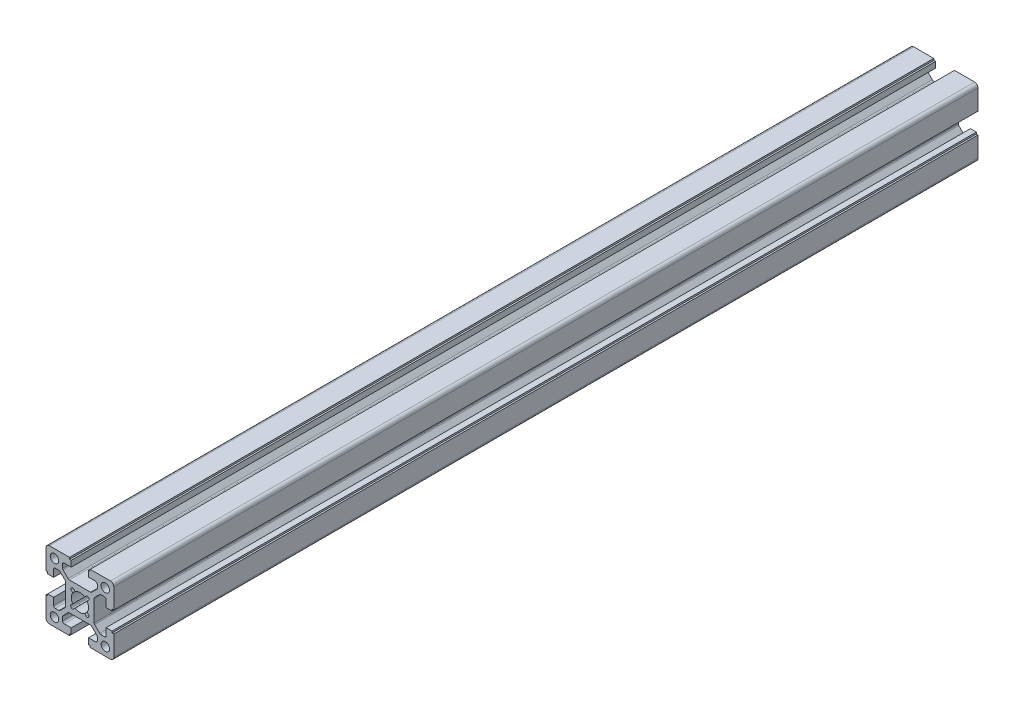
from build123d import *

# Parameters (mm, degrees)
SKETCH1_R           = 2.5
BOSS_EXTRUDE1_DEPTH = 255


with BuildPart() as part:
    # Sketch1 → Boss-Extrude1 (new, symmetric)
    with BuildSketch(Plane.XY):
        with BuildLine():
            Line((-5.1005, 15.500896213), (-5.1005, 19.000896213))
            Line((-5.1005, 19.000896213), (-6.1005, 19.000896213))
            Line((-6.1005, 19.000896213), (-6.1005, 20.000896213))
            Line((-6.1005, 20.000896213), (-18.0005, 20.000896213))
            ThreePointArc((-18.0005, 20.000896213), (-19.414713562, 19.415109775), (-20.0005, 18.000896213))
            Line((-20.0005, 18.000896213), (-20.0005, 6.100896213))
            Line((-20.0005, 6.100896213), (-19.0005, 6.100896213))
            Line((-19.0005, 6.100896213), (-19.0005, 5.100896213))
            Line((-19.0005, 5.100896213), (-15.5005, 5.100896213))
            Line((-15.5005, 5.100896213), (-15.5005, 9.250896213))
            ThreePointArc((-15.5005, 9.250896213), (-15.207606781, 9.958002994), (-14.5005, 10.250896213))
            Line((-14.5005, 10.250896213), (-12.431713562, 10.250896213))
            ThreePointArc((-12.431713562, 10.250896213), (-12.049030228, 10.174775786), (-11.724606932, 9.958003144))
            Line((-11.724606932, 9.958003144), (-8.693393219, 6.926789431))
            ThreePointArc((-8.693393219, 6.926789431), (-8.476620546, 6.602366272), (-8.4005, 6.21968306))
            Line((-8.4005, 6.21968306), (-8.4005, -6.217890225))
            ThreePointArc((-8.4005, -6.217890225), (-8.476620502, -6.60057374), (-8.693393346, -6.924997133))
            Line((-8.693393346, -6.924997133), (-11.724606781, -9.956210569))
            ThreePointArc((-11.724606781, -9.956210569), (-12.049030198, -10.172983348), (-12.431713709, -10.249103787))
            Line((-12.431713709, -10.249103787), (-14.5005, -10.249103787))
            ThreePointArc((-14.5005, -10.249103787), (-15.207606781, -9.956210569), (-15.5005, -9.249103787))
            Line((-15.5005, -9.249103787), (-15.5005, -5.099103787))
            Line((-15.5005, -5.099103787), (-19.0005, -5.099103787))
            Line((-19.0005, -5.099103787), (-19.0005, -6.099103787))
            Line((-19.0005, -6.099103787), (-20.0005, -6.099103787))
            Line((-20.0005, -6.099103787), (-20.0005, -17.999103787))
            ThreePointArc((-20.0005, -17.999103787), (-19.414713562, -19.41331735), (-18.0005, -19.999103787))
            Line((-18.0005, -19.999103787), (-6.1005, -19.999103787))
            Line((-6.1005, -19.999103787), (-6.1005, -18.999103787))
            Line((-6.1005, -18.999103787), (-5.1005, -18.999103787))
            Line((-5.1005, -18.999103787), (-5.1005, -15.499103787))
            Line((-5.1005, -15.499103787), (-9.2505, -15.499103787))
            ThreePointArc((-9.2505, -15.499103787), (-9.957606781, -15.206210569), (-10.2505, -14.499103787))
            Line((-10.2505, -14.499103787), (-10.2505, -12.43131735))
            ThreePointArc((-10.2505, -12.43131735), (-10.174379535, -12.048633922), (-9.957606789, -11.724210576))
            Line((-9.957606789, -11.724210576), (-6.925393219, -8.691997006))
            ThreePointArc((-6.925393219, -8.691997006), (-6.60096987, -8.475224255), (-6.218286438, -8.399103787))
            Line((-6.218286438, -8.399103787), (6.218286438, -8.399103787))
            ThreePointArc((6.218286438, -8.399103787), (6.600969772, -8.475224214), (6.925393068, -8.691996856))
            Line((6.925393068, -8.691996856), (9.956606781, -11.723210569))
            ThreePointArc((9.956606781, -11.723210569), (10.173379454, -12.047633728), (10.2495, -12.43031694))
            Line((10.2495, -12.43031694), (10.2495, -14.499103787))
            ThreePointArc((10.2495, -14.499103787), (9.956606781, -15.206210569), (9.2495, -15.499103787))
            Line((9.2495, -15.499103787), (5.0995, -15.499103787))
            Line((5.0995, -15.499103787), (5.0995, -18.999103787))
            Line((5.0995, -18.999103787), (6.0995, -18.999103787))
            Line((6.0995, -18.999103787), (6.0995, -19.999103787))
            Line((6.0995, -19.999103787), (17.9995, -19.999103787))
            ThreePointArc((17.9995, -19.999103787), (19.413713562, -19.41331735), (19.9995, -17.999103787))
            Line((19.9995, -17.999103787), (19.9995, -6.099103787))
            Line((19.9995, -6.099103787), (18.9995, -6.099103787))
            Line((18.9995, -6.099103787), (18.9995, -5.099103787))
            Line((18.9995, -5.099103787), (15.4995, -5.099103787))
            Line((15.4995, -5.099103787), (15.4995, -9.249103787))
            ThreePointArc((15.4995, -9.249103787), (15.206606781, -9.956210569), (14.4995, -10.249103787))
            Line((14.4995, -10.249103787), (12.431713562, -10.249103787))
            ThreePointArc((12.431713562, -10.249103787), (12.049030135, -10.172983322), (11.724606789, -9.956210576))
            Line((11.724606789, -9.956210576), (8.692393219, -6.923997006))
            ThreePointArc((8.692393219, -6.923997006), (8.475620467, -6.599573657), (8.3995, -6.216890225))
            Line((8.3995, -6.216890225), (8.3995, 6.21868265))
            ThreePointArc((8.3995, 6.21868265), (8.475620465, 6.601366078), (8.692393211, 6.925789424))
            Line((8.692393211, 6.925789424), (11.724606781, 9.958002994))
            ThreePointArc((11.724606781, 9.958002994), (12.04903013, 10.174775745), (12.431713562, 10.250896213))
            Line((12.431713562, 10.250896213), (14.4995, 10.250896213))
            ThreePointArc((14.4995, 10.250896213), (15.206606781, 9.958002994), (15.4995, 9.250896213))
            Line((15.4995, 9.250896213), (15.4995, 5.100896213))
            Line((15.4995, 5.100896213), (18.9995, 5.100896213))
            Line((18.9995, 5.100896213), (18.9995, 6.100896213))
            Line((18.9995, 6.100896213), (19.9995, 6.100896213))
            Line((19.9995, 6.100896213), (19.9995, 18.000896213))
            ThreePointArc((19.9995, 18.000896213), (19.413713562, 19.415109775), (17.9995, 20.000896213))
            Line((17.9995, 20.000896213), (6.0995, 20.000896213))
            Line((6.0995, 20.000896213), (6.0995, 19.000896213))
            Line((6.0995, 19.000896213), (5.0995, 19.000896213))
            Line((5.0995, 19.000896213), (5.0995, 15.500896213))
            Line((5.0995, 15.500896213), (9.2495, 15.500896213))
            ThreePointArc((9.2495, 15.500896213), (9.956606781, 15.208002994), (10.2495, 14.500896213))
            Line((10.2495, 14.500896213), (10.2495, 12.432109775))
            ThreePointArc((10.2495, 12.432109775), (10.173379498, 12.04942626), (9.956606654, 11.725002867))
            Line((9.956606654, 11.725002867), (6.925393219, 8.693789431))
            ThreePointArc((6.925393219, 8.693789431), (6.600969802, 8.477016652), (6.218286291, 8.400896213))
            Line((6.218286291, 8.400896213), (-6.218286438, 8.400896213))
            ThreePointArc((-6.218286438, 8.400896213), (-6.600969865, 8.477016678), (-6.925393211, 8.693789424))
            Line((-6.925393211, 8.693789424), (-9.957606781, 11.726002994))
            ThreePointArc((-9.957606781, 11.726002994), (-10.174379533, 12.050426343), (-10.2505, 12.433109775))
            Line((-10.2505, 12.433109775), (-10.2505, 14.500896213))
            ThreePointArc((-10.2505, 14.500896213), (-9.957606781, 15.208002994), (-9.2505, 15.500896213))
            Line((-9.2505, 15.500896213), (-5.1005, 15.500896213))
        make_face()
        with Locations((-15.0005, 15.000896213)):
            Circle(SKETCH1_R, mode=Mode.SUBTRACT)
        with Locations((14.9995, -14.999103787)):
            Circle(SKETCH1_R, mode=Mode.SUBTRACT)
        with Locations((-15.0005, -14.999103787)):
            Circle(SKETCH1_R, mode=Mode.SUBTRACT)
        with Locations((14.9995, 15.000896213)):
            Circle(SKETCH1_R, mode=Mode.SUBTRACT)
        with BuildLine():
            Line((-5.179163629, 3.765559841), (-4.2435, 2.829896213))
            ThreePointArc((-4.2435, 2.829896213), (-5.100062832, 0.000896213), (-4.2435, -2.828103787))
            Line((-4.2435, -2.828103787), (-5.277169914, -3.861773701))
            ThreePointArc((-5.277169914, -3.861773701), (-5.496839828, -4.392103787), (-5.277169914, -4.922433873))
            Line((-5.277169914, -4.922433873), (-4.923994614, -5.275609174))
            ThreePointArc((-4.923994614, -5.275609174), (-4.393905685, -5.495279049), (-3.8636756, -5.275950112))
            Line((-3.8636756, -5.275950112), (-2.8295, -4.243103787))
            ThreePointArc((-2.8295, -4.243103787), (0, -5.1), (2.8295, -4.243103787))
            Line((2.8295, -4.243103787), (3.778597046, -5.192200834))
            ThreePointArc((3.778597046, -5.192200834), (4.308685975, -5.411870709), (4.83891606, -5.192541772))
            Line((4.83891606, -5.192541772), (5.192983438, -4.838929494))
            ThreePointArc((5.192983438, -4.838929494), (5.412994471, -4.308499627), (5.193324596, -3.777928383))
            Line((5.193324596, -3.777928383), (4.2435, -2.828103787))
            ThreePointArc((4.2435, -2.828103787), (5.100062832, 0.000896213), (4.2435, 2.829896213))
            Line((4.2435, 2.829896213), (5.193264407, 3.77966062))
            ThreePointArc((5.193264407, 3.77966062), (5.412934321, 4.309990706), (5.193264407, 4.840320791))
            Line((5.193264407, 4.840320791), (4.839313907, 5.194271291))
            ThreePointArc((4.839313907, 5.194271291), (4.308742664, 5.413941166), (3.778312797, 5.193930133))
            Line((3.778312797, 5.193930133), (2.8295, 4.243896213))
            ThreePointArc((2.8295, 4.243896213), (0, 5.100792425), (-2.8295, 4.243896213))
            Line((-2.8295, 4.243896213), (-3.765163629, 5.179559841))
            ThreePointArc((-3.765163629, 5.179559841), (-4.295493715, 5.399229756), (-4.825823801, 5.179559841))
            Line((-4.825823801, 5.179559841), (-5.179163629, 4.826220013))
            ThreePointArc((-5.179163629, 4.826220013), (-5.398833543, 4.295889927), (-5.179163629, 3.765559841))
        make_face(mode=Mode.SUBTRACT)
    extrude(amount=BOSS_EXTRUDE1_DEPTH, both=True)


solid = part.part
